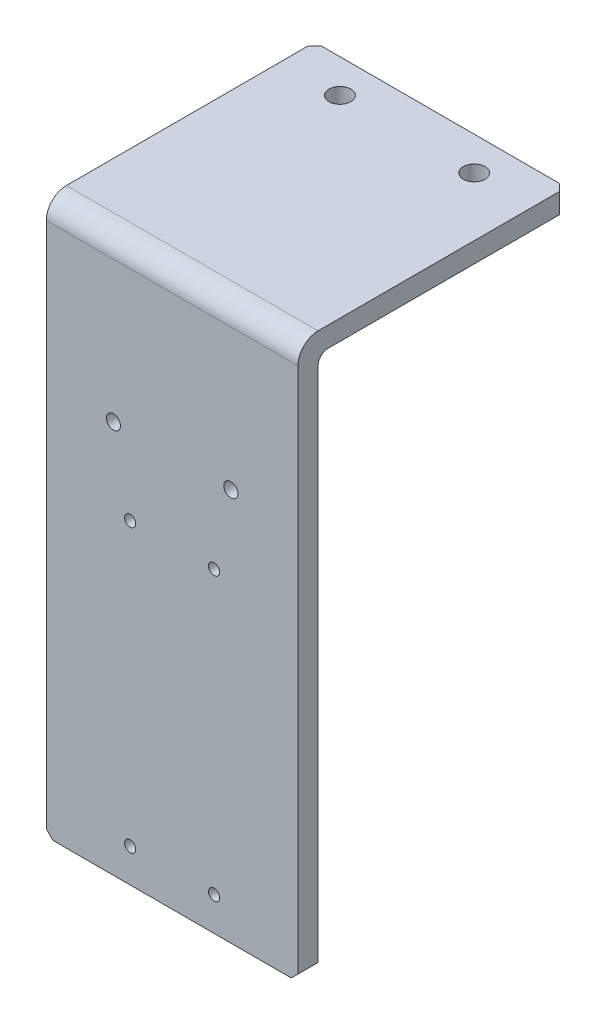
SolidWorks part; units mm, degrees
material "SPCC"
ref_plane "Front Plane" through (0, 0, 0) normal (0, 0, 1) x (1, 0, 0)
ref_plane "Top Plane" through (0, 0, 0) normal (0, 1, 0) x (1, 0, 0)
ref_plane "Right Plane" through (0, 0, 0) normal (1, 0, 0) x (0, 0, -1)
sketch "Sketch1" plane through (0, 0, 0) normal (0, 0, 1) x (1, 0, 0)
  line L1 (-37.5, 82.5) -> (37.5, 82.5)
  line L2 (-37.5, 82.5) -> (-37.5, -82.5)
  line L3 (-37.5, -82.5) -> (37.5, -82.5)
  line L4 (37.5, 82.5) -> (37.5, -82.5)
  line L5 (-37.5, 82.5) -> (37.5, -82.5) construction
  line L6 (-37.5, -82.5) -> (37.5, 82.5) construction
  point P0 (0, 0)
  dimension "D1" = 75
  dimension "D2" = 165
extrude "Boss-Extrude1" add sketch "Sketch1" along normal blind 80
shell "Shell1" thickness 6
fillet "Fillet1" radius 6 1 edges at (0, 82.5, 80)
fillet "Fillet2" radius 3 1 edges at (0, 76.5, 74)
chamfer "Chamfer1" distance 2 angle 45 4 edges at (37.5, -82.5, 77) (-37.5, -82.5, 77) (-37.5, 79.5, 0) (37.5, 79.5, 0)
hole_wizard "M4 Tapped Hole1" positions "Sketch3" profile "Sketch2" tap size "M4" standard "GB" end condition through all
sketch "Sketch3" plane through (0, 0, 74) normal (0, 0, -1) x (-1, 0, 0)
  line L0 (0, 0) -> (0, 72.9265) construction
  line L1 (35.5, -82.5) -> (-35.5, -82.5) construction
  point P0 (-12.5, -72.5)
  point P4 (-12.5, 11.5)
  point P15 (12.5, 11.5)
  point P16 (12.5, -72.5)
  dimension "D1" = 84
  dimension "D2" = 10
  dimension "D3" = 25
  dimension "D4" = 25
cosmetic thread "Cosmetic Thread1" parameters "D2"=4
cosmetic thread "Cosmetic Thread2" parameters "D2"=4
cosmetic thread "Cosmetic Thread3" parameters "D2"=4
cosmetic thread "Cosmetic Thread4" parameters "D2"=4
sketch "Sketch2" plane through (12.5, -72.5, 74) normal (1, 0, 0) x (0, 1, 0)
  line L0 (0, 0) -> (0, 6)
  line L1 (0, 6) -> (1.65, 6)
  line L2 (1.65, 6) -> (1.65, 0)
  line L5 (1.65, 0) -> (0, 0)
  line L11 (0, -6.35) -> (0, 107.95) construction
  dimension "通孔螺纹孔钻头直径" = 3.3
  dimension "通孔螺纹孔钻头深度" = 6
hole_wizard "Ø6.5 (6.5) Diameter Hole1" positions "Sketch5" profile "Sketch4" hole size "Ø6.5" standard "GB"
sketch "Sketch5" plane through (0, 76.5, 0) normal (0, -1, 0) x (1, 0, 0)
  line L0 (0, 0) -> (0, 25.3791) construction
  line L1 (35.5, 0) -> (-35.5, 0) construction
  point P0 (-20, 10)
  point P6 (20, 10)
  dimension "D1" = 40
  dimension "D2" = 10
sketch "Sketch4" plane through (-20, 76.5, 10) normal (1, 0, 0) x (0, 0, -1)
  line L0 (0, 0) -> (0, 11.9528)
  line L1 (0, 11.9528) -> (3.25, 10)
  line L2 (3.25, 10) -> (3.25, 0)
  line L5 (3.25, 0) -> (0, 0)
  line L10 (0, 11.9528) -> (-3.25, 10) construction
  line L11 (0, -6.35) -> (0, 107.95) construction
  dimension "孔直径" = 6.5
  dimension "孔深度" = 10
  dimension "导头角度" = 118
hole_wizard "M5 Tapped Hole1" positions "Sketch7" profile "Sketch8" tap size "M5" standard "GB" end condition through all
sketch "Sketch7" plane through (0, 0, 74) normal (0, 0, -1) x (-1, 0, 0)
  line L0 (0, 0) -> (0, 26.5768) construction
  point P0 (-17.5, 34.5)
  point P10 (17.5, 34.5)
  dimension "D2" = 34.5
  dimension "D1" = 17.5
sketch "Sketch8" plane through (17.5, 34.5, 74) normal (1, 0, 0) x (0, 1, 0)
  line L0 (0, 0) -> (0, 6)
  line L1 (0, 6) -> (2.1, 6)
  line L2 (2.1, 6) -> (2.1, 0)
  line L5 (2.1, 0) -> (0, 0)
  line L11 (0, -6.35) -> (0, 107.95) construction
  dimension "通孔螺纹孔钻头直径" = 4.2
  dimension "通孔螺纹孔钻头深度" = 6
cosmetic thread "Cosmetic Thread5" parameters "D2"=5
cosmetic thread "Cosmetic Thread6" parameters "D2"=5
